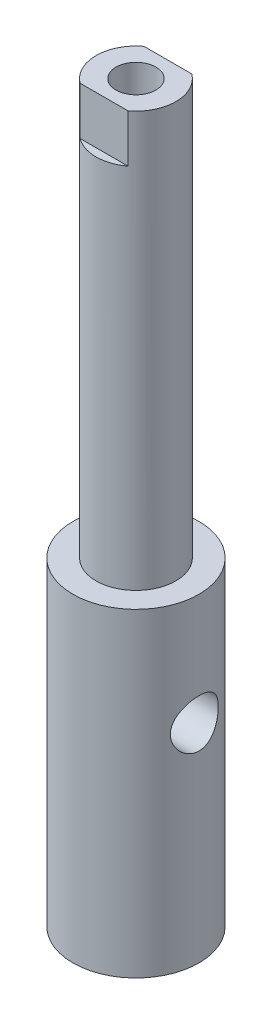
SolidWorks part; units mm, degrees
ref_plane "Front Plane" through (0, 0, 0) normal (0, 0, 1) x (1, 0, 0)
ref_plane "Top Plane" through (0, 0, 0) normal (0, 1, 0) x (1, 0, 0)
ref_plane "Right Plane" through (0, 0, 0) normal (1, 0, 0) x (0, 0, -1)
sketch "Sketch1" plane through (0, 0, 0) normal (0, 1, 0) x (1, 0, 0)
  circle A0 centre (0, 0) radius 3.95
  dimension "D1" = 7.9
extrude "Boss-Extrude1" add sketch "Sketch1" along normal blind 20
sketch "Sketch2" plane through (0, 20, 0) normal (0, 1, 0) x (1, 0, 0)
  circle A0 centre (0, 0) radius 2.5
  dimension "D1" = 5
extrude "Boss-Extrude2" add sketch "Sketch2" along normal blind 26
sketch "Sketch3" plane through (0, 46, 0) normal (0, 1, 0) x (1, 0, 0)
  line L1 (-2.898, 2) -> (2.898, 2)
  line L2 (-2.898, 2) -> (-2.898, -2)
  line L3 (-2.898, -2) -> (2.898, -2)
  line L4 (2.898, 2) -> (2.898, -2)
  line L5 (-2.898, 2) -> (2.898, -2) construction
  line L6 (-2.898, -2) -> (2.898, 2) construction
  point P0 (0, 0)
  dimension "D1" = 4
extrude "Cut-Extrude1" cut sketch "Sketch3" against normal blind 3 flip side to cut
sketch "Sketch4" plane through (0, 0, 0) normal (1, 0, 0) x (0, 0, -1)
  circle A0 centre (0, 13) radius 1.5
  dimension "D1" = 3
  dimension "D2" = 13
extrude "Cut-Extrude2" cut sketch "Sketch4" against normal through all both and the other way through all
sketch "Sketch5" plane through (0, 0, 0) normal (1, 0, 0) x (0, 0, -1)
  circle A0 centre (0, 13) radius 2
  dimension "4.5" = 4
extrude "Cut-Extrude3" cut sketch "Sketch5" against normal blind 10 from offset 1.5 offset against normal yes
hole_wizard "M3 Tapped Hole2" positions "3DSketch1" profile "Sketch6" tap size "M3" standard "GB"
sketch3d "3DSketch1"
  arc A0 (-1.5, 46, -2) -> (-1.5, 46, 2) centre (0, 46, 0) ccw construction
  point P0 (0, 0, 0)
  point P4 (0, 46, 0)
  point P11 (0, 48.5, 0)
sketch "Sketch6" plane through (0, 46, 0) normal (1, 0, 0) x (0, 0, 1)
  line L0 (0, 0) -> (0, 8.2511)
  line L1 (0, 8.2511) -> (1.25, 7.5)
  line L2 (1.25, 7.5) -> (1.25, 0)
  line L5 (1.25, 0) -> (0, 0)
  line L10 (0, 8.2511) -> (-1.25, 7.5) construction
  line L11 (0, -6.35) -> (0, 107.95) construction
  dimension "螺纹孔钻头直径" = 2.5
  dimension "螺纹孔钻头深度" = 7.5
  dimension "导头角度" = 118
cosmetic thread "Hole thread 3" parameters "D1"=6, "D2"=3
cosmetic thread "Hole thread 4" parameters "D1"=6, "D2"=3
